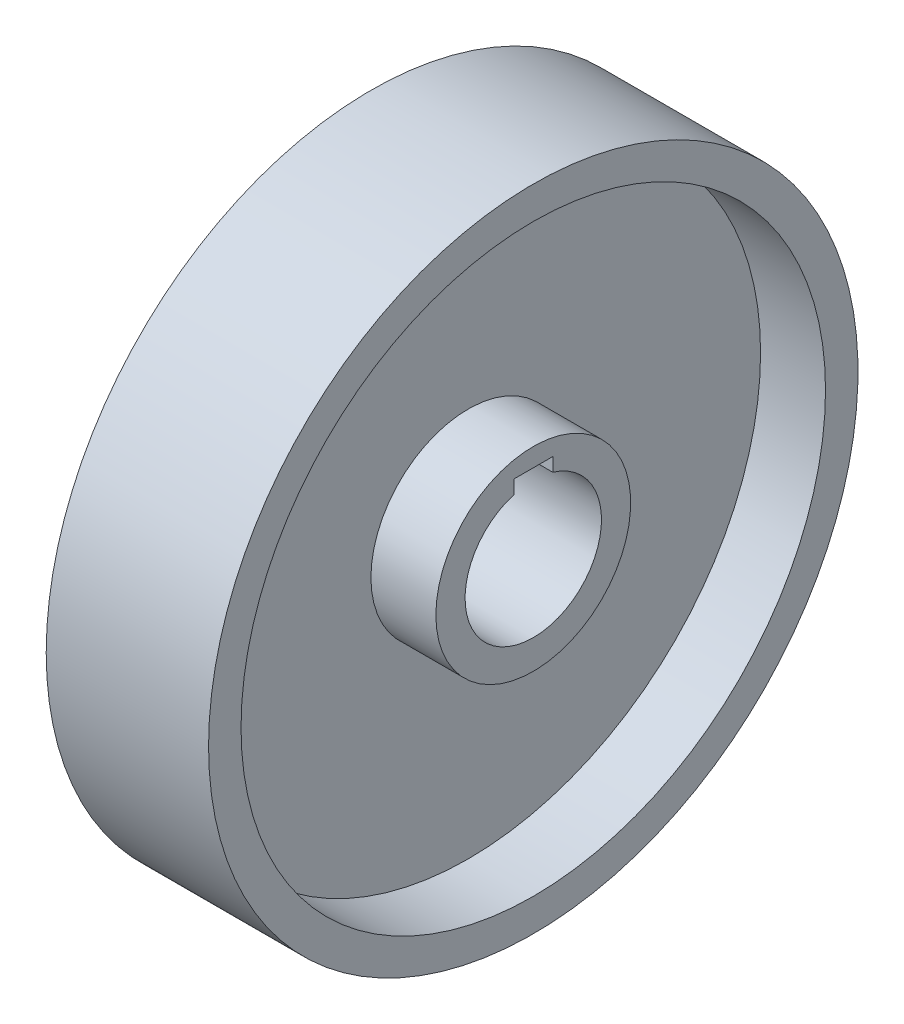
SolidWorks part; units mm, degrees
material "Q235B"
ref_plane "Front Plane" through (0, 0, 0) normal (0, 0, 1) x (1, 0, 0)
ref_plane "Top Plane" through (0, 0, 0) normal (0, 1, 0) x (1, 0, 0)
ref_plane "Right Plane" through (0, 0, 0) normal (1, 0, 0) x (0, 0, -1)
sketch "Sketch1" plane through (0, 0, 0) normal (0, 0, 1) x (1, 0, 0)
  line L0 (-25, 21) -> (25, 21)
  line L1 (25, 21) -> (25, 30)
  line L2 (25, 30) -> (5, 30)
  line L3 (5, 30) -> (5, 90)
  line L4 (5, 90) -> (25, 90)
  line L5 (25, 90) -> (25, 100)
  line L6 (25, 100) -> (-25, 100)
  line L7 (0, 100) -> (0, 21) construction
  line L8 (-25, 90) -> (-25, 100)
  line L9 (-5, 90) -> (-25, 90)
  line L10 (-5, 30) -> (-5, 90)
  line L11 (-25, 30) -> (-5, 30)
  line L12 (-25, 21) -> (-25, 30)
  line L13 (0, 0) -> (38.5179, 0) construction
  dimension "D1" = 200
  dimension "D2" = 50
  dimension "D3" = 42
  dimension "D4" = 10
  dimension "D5" = 10
  dimension "D6" = 60
revolve "Revolve1" add sketch "Sketch1" angle 360 about L13
sketch "Sketch2" plane through (25, 0, 0) normal (1, 0, 0) x (0, 0, -1)
  line L1 (6, 17.7) -> (-6, 17.7)
  line L2 (6, 17.7) -> (6, 24.3)
  line L3 (6, 24.3) -> (-6, 24.3)
  line L4 (-6, 17.7) -> (-6, 24.3)
  line L5 (6, 17.7) -> (-6, 24.3) construction
  line L6 (6, 24.3) -> (-6, 17.7) construction
  circle A0 centre (0, 0) radius 21 construction
  point P0 (0, 21)
  dimension "D1" = 12
  dimension "D2" = 45.3
extrude "Cut-Extrude1" cut sketch "Sketch2" against normal up to next
